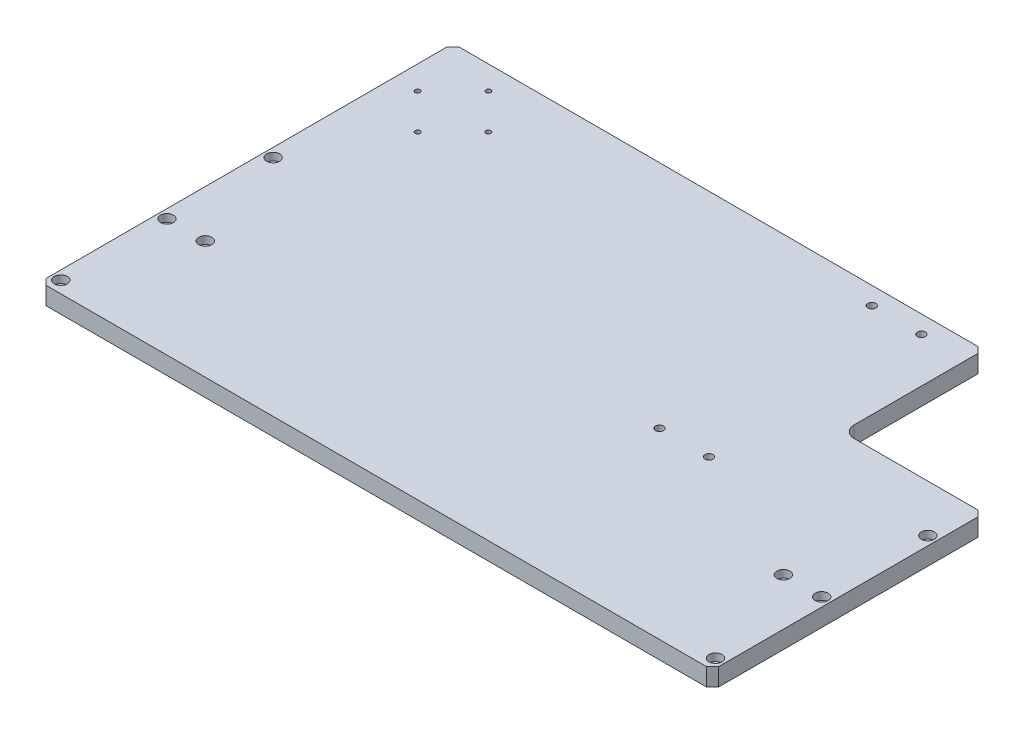
SolidWorks part; units mm, degrees
material "6061"
ref_plane "前视基准面" through (0, 0, 0) normal (0, 0, 1) x (1, 0, 0)
ref_plane "上视基准面" through (0, 0, 0) normal (0, 1, 0) x (1, 0, 0)
ref_plane "右视基准面" through (0, 0, 0) normal (1, 0, 0) x (0, 0, -1)
sketch "草图1" plane through (0, 0, 0) normal (0, 1, 0) x (1, 0, 0)
  line L1 (285, -175) -> (-285, -175)
  line L2 (285, -175) -> (285, 175)
  line L3 (285, 175) -> (-285, 175)
  line L4 (-285, -175) -> (-285, 175)
  line L5 (285, -175) -> (-285, 175) construction
  line L6 (285, 175) -> (-285, -175) construction
  point P0 (0, 0)
  dimension "D1" = 570
  dimension "D2" = 350
extrude "凸台-拉伸1" add sketch "草图1" along normal mid plane 15
chamfer "倒角1" distance 5 angle 45 4 edges at (285, 0, -175) (285, 0, 175) (-285, 0, -175) (-285, 0, 175)
hole_wizard "M5 螺纹孔1" positions "草图2" profile "草图3" tap size "M5" standard "GB" end condition through all
sketch "草图2" plane through (0, 7.5, 0) normal (0, 1, 0) x (1, 0, 0)
  point P0 (-265, 125)
  point P3 (-235, 95)
  point P6 (-235, 155)
  point P9 (-205, 125)
sketch "草图3" plane through (-265, 7.5, -125) normal (1, 0, 0) x (0, 0, 1)
  line L0 (0, 0) -> (0, 15)
  line L1 (0, 15) -> (2.1, 15)
  line L2 (2.1, 15) -> (2.1, 0)
  line L5 (2.1, 0) -> (0, 0)
  line L11 (0, -6.35) -> (0, 107.95) construction
  dimension "通孔螺纹孔钻头直径" = 4.2
  dimension "通孔螺纹孔钻头深度" = 15
cosmetic thread "孔螺蚊线9" parameters "D2"=5
cosmetic thread "孔螺蚊线11" parameters "D2"=5
cosmetic thread "孔螺蚊线12" parameters "D2"=5
cosmetic thread "孔螺蚊线13" parameters "D2"=5
hole_wizard "M8 螺纹孔1" positions "草图4" profile "草图5" tap size "M8" standard "ISO" end condition through all
sketch "草图4" plane through (0, 7.5, 0) normal (0, 1, 0) x (1, 0, 0)
  point P0 (85, -20)
  point P3 (127, -20)
  point P6 (127, 160)
  point P9 (85, 160)
sketch "草图5" plane through (85, 7.5, 20) normal (1, 0, 0) x (0, 0, 1)
  line L0 (0, 0) -> (0, 15)
  line L1 (0, 15) -> (3.4, 15)
  line L2 (3.4, 15) -> (3.4, 0)
  line L5 (3.4, 0) -> (0, 0)
  line L11 (0, -6.35) -> (0, 107.95) construction
  dimension "通孔螺纹孔钻头直径" = 6.8
  dimension "通孔螺纹孔钻头深度" = 15
cosmetic thread "孔螺蚊线5" parameters "D2"=8
cosmetic thread "孔螺蚊线6" parameters "D2"=8
cosmetic thread "孔螺蚊线7" parameters "D2"=8
cosmetic thread "孔螺蚊线8" parameters "D2"=8
hole_wizard "M6 六角凹头螺钉的柱形沉头孔1" positions "草图6" profile "草图7" counterbore size "M6" standard "ISO"
sketch "草图6" plane through (0, 7.5, 0) normal (0, 1, 0) x (1, 0, 0)
  line L1 (-277.5, 15) -> (277.5, 15)
  line L2 (-277.5, 15) -> (-277.5, -165)
  line L3 (-277.5, -165) -> (277.5, -165)
  line L4 (277.5, 15) -> (277.5, -165)
  line L6 (-280, -175) -> (280, -175) construction
  line L7 (0, 103.6386) -> (0, -261.2443) construction
  point P0 (-277.5, 15)
  point P2 (-277.5, -165)
  point P4 (277.5, 15)
  point P6 (277.5, -165)
  point P246 (-277.5, -75)
  point P248 (277.5, -75)
  dimension "D1" = 555
  dimension "D2" = 180
  dimension "D3" = 10
sketch "草图7" plane through (-277.5, 7.5, -15) normal (1, 0, 0) x (0, 0, 1)
  line L0 (0, 0) -> (0, 18.9828)
  line L1 (0, 18.9828) -> (3.3, 17)
  line L2 (3.3, 17) -> (3.3, 6.4)
  line L3 (3.3, 6.4) -> (5.5, 6.4)
  line L4 (5.5, 6.4) -> (5.5, 0)
  line L5 (5.5, 0) -> (0, 0)
  line L10 (0, 18.9828) -> (-3.3, 17) construction
  line L11 (0, -6.35) -> (0, 107.95) construction
  dimension "孔直径" = 6.6
  dimension "孔深度" = 17
  dimension "柱形沉头孔直径" = 11
  dimension "柱形沉头孔深度" = 6.4
  dimension "导头角度" = 118
hole_wizard "M6 六角凹头螺钉的柱形沉头孔2" positions "草图8" profile "草图9" counterbore size "M6" standard "ISO"
sketch "草图8" plane through (0, 7.5, 0) normal (0, 1, 0) x (1, 0, 0)
  line L3 (0, -175) -> (0, 132.1449) construction
  line L4 (-280, -175) -> (280, -175) construction
  line L5 (245, -75) -> (-245, -75) construction
  point P0 (-245, -75)
  point P2 (245, -75)
  dimension "D1" = 490
  dimension "D2" = 100
sketch "草图9" plane through (-245, 7.5, 75) normal (1, 0, 0) x (0, 0, 1)
  line L0 (0, 0) -> (0, 18.9828)
  line L1 (0, 18.9828) -> (3.3, 17)
  line L2 (3.3, 17) -> (3.3, 6.4)
  line L3 (3.3, 6.4) -> (5.5, 6.4)
  line L4 (5.5, 6.4) -> (5.5, 0)
  line L5 (5.5, 0) -> (0, 0)
  line L10 (0, 18.9828) -> (-3.3, 17) construction
  line L11 (0, -6.35) -> (0, 107.95) construction
  dimension "孔直径" = 6.6
  dimension "孔深度" = 17
  dimension "柱形沉头孔直径" = 11
  dimension "柱形沉头孔深度" = 6.4
  dimension "导头角度" = 118
sketch "草图10" plane through (0, 7.5, 0) normal (0, 1, 0) x (1, 0, 0)
  line L0 (285, -170) -> (285, 170) construction
  line L1 (285, 175) -> (165, 175)
  line L2 (285, 175) -> (285, 55)
  line L3 (285, 55) -> (165, 55)
  line L4 (165, 175) -> (165, 55)
  line L5 (280, 175) -> (-280, 175) construction
  dimension "D1" = 120
extrude "切除-拉伸1" cut sketch "草图10" against normal through all
fillet "圆角1" radius 10 1 edges at (165, 0, -55)
chamfer "倒角2" distance 5 angle 45 2 edges at (165, 0, -175) (285, 0, -55)
